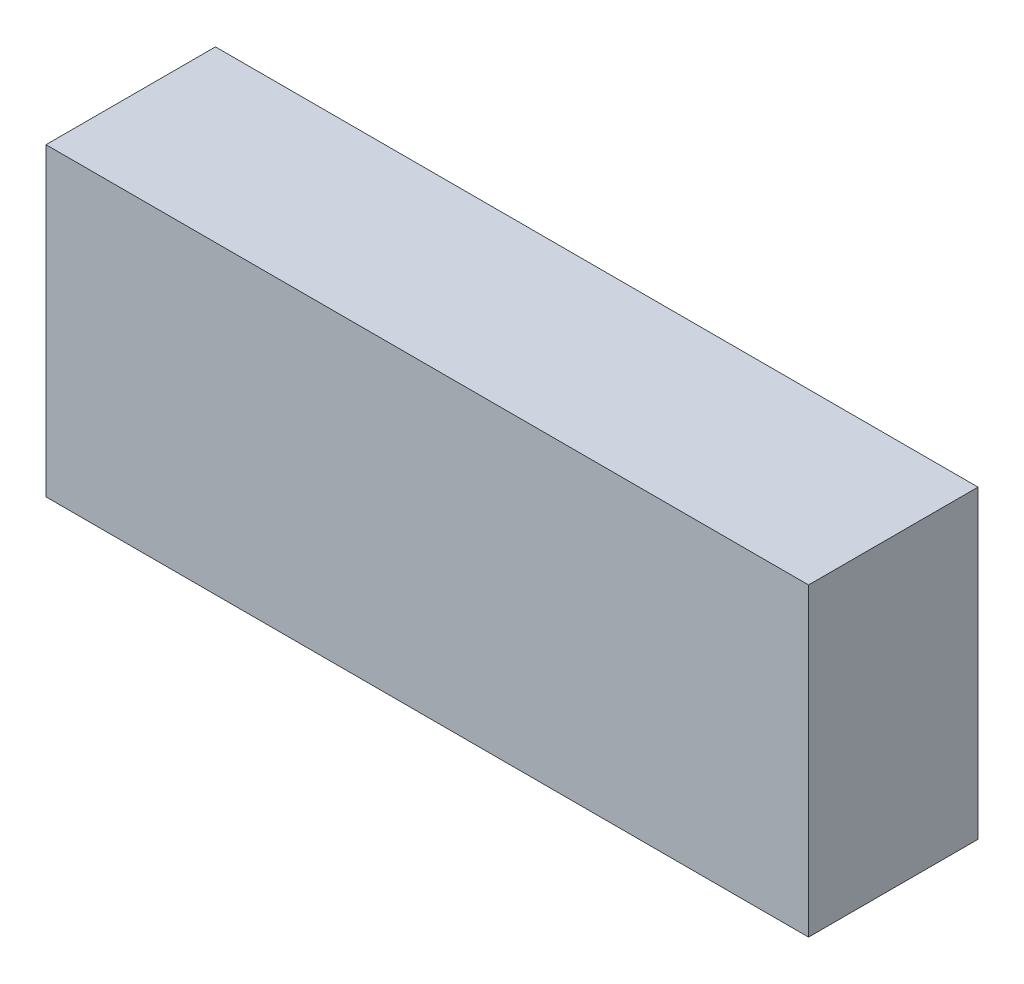
from build123d import *

# Parameters (mm, degrees)
SKETCH_1_W      = 45
SKETCH_1_H      = 18
EXTRUDE_1_DEPTH = 5


with BuildPart() as part:
    # 草图1 → 凸台-拉伸1 (new, symmetric)
    with BuildSketch(Plane.XY):
        Rectangle(SKETCH_1_W, SKETCH_1_H)
    extrude(amount=EXTRUDE_1_DEPTH, both=True)


solid = part.part
